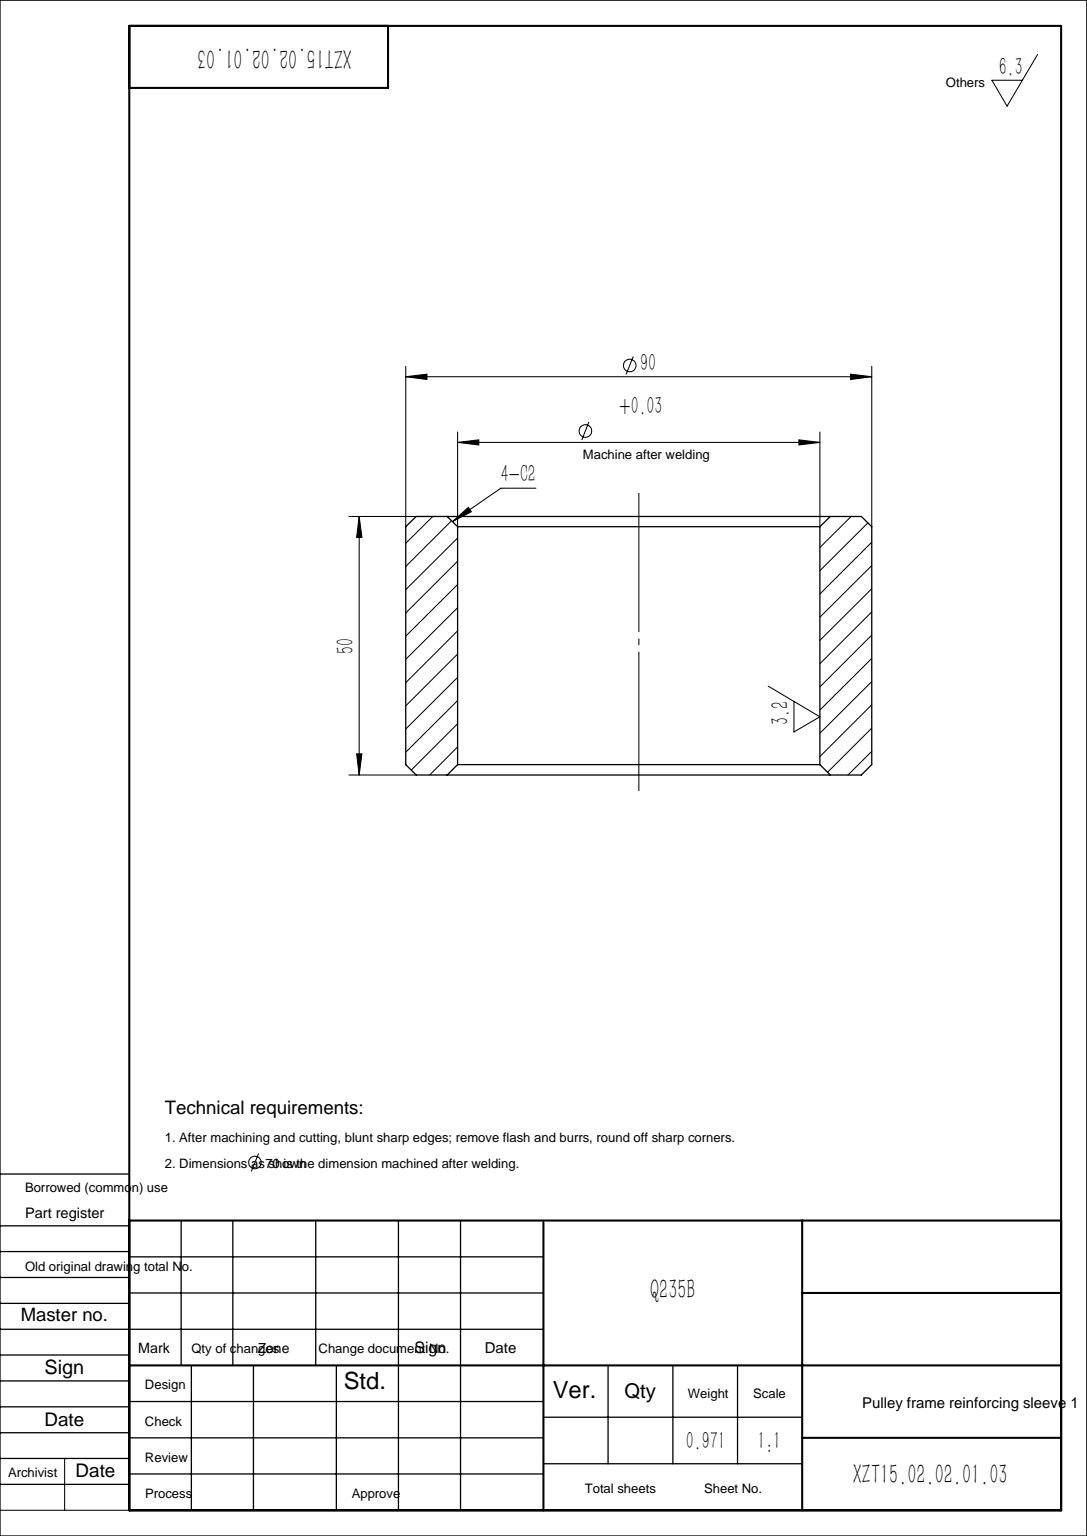
from build123d import *

# Parameters (mm, degrees)
SKETCH1_R           = 45
SKETCH1_R_2         = 35
BOSS_EXTRUDE1_DEPTH = 50
CHAMFER2_SIZE       = 2


with BuildPart() as part:
    # Sketch1 → Boss-Extrude1 (new body)
    with BuildSketch(Plane(origin=(0, 0, 0), x_dir=(1, 0, 0), z_dir=(0, 1, 0))):
        with Locations(Location((0, 0, 0), (0, 0, 270))):
            Circle(SKETCH1_R)
        with Locations(Location((0, 0, 0), (0, 0, 270))):
            Circle(SKETCH1_R_2, mode=Mode.SUBTRACT)
    extrude(amount=BOSS_EXTRUDE1_DEPTH)

    # Chamfer2
    chamfer2_edges = [part.edges().sort_by_distance(p)[0] for p in [
        (0, 0, -45),
        (0, 50, -45),
        (0, 0, -35),
        (0, 50, -35),
    ]]
    chamfer(chamfer2_edges, length=CHAMFER2_SIZE)


solid = part.part
